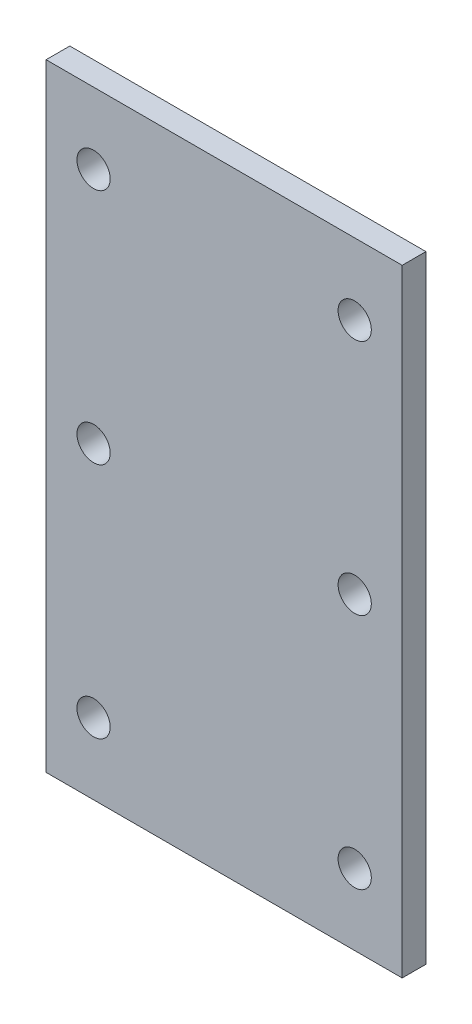
SolidWorks part; units mm, degrees
material "Q235B"
ref_plane "Front Plane" through (0, 0, 0) normal (0, 0, 1) x (1, 0, 0)
ref_plane "Top Plane" through (0, 0, 0) normal (0, 1, 0) x (1, 0, 0)
ref_plane "Right Plane" through (0, 0, 0) normal (1, 0, 0) x (0, 0, -1)
sketch "Sketch1" plane through (0, 0, 0) normal (0, 0, 1) x (1, 0, 0)
  line L1 (75, -130) -> (-75, -130)
  line L2 (75, -130) -> (75, 130)
  line L3 (75, 130) -> (-75, 130)
  line L4 (-75, -130) -> (-75, 130)
  line L5 (75, -130) -> (-75, 130) construction
  line L6 (75, 130) -> (-75, -130) construction
  point P0 (0, 0)
  dimension "D1" = 260
  dimension "D2" = 150
extrude "Boss-Extrude1" add sketch "Sketch1" along normal blind 10
hole_wizard "Ø14.0 (14) Diameter Hole1" positions "Sketch2" profile "Sketch3" hole size "Ø14.0" standard "GB" end condition up to next
sketch "Sketch2" plane through (0, 0, 10) normal (0, 0, 1) x (1, 0, 0)
  line L0 (0, 60.7971) -> (0, 0) construction
  line L1 (0, 0) -> (-55, 0) construction
  line L3 (75, 130) -> (-75, 130) construction
  point P0 (-55, 100)
  point P2 (-55, 0)
  point P15 (-55, -100)
  point P16 (55, -100)
  point P17 (55, 0)
  point P18 (55, 100)
  dimension "D1" = 110
  dimension "D2" = 30
sketch "Sketch3" plane through (-55, 100, 10) normal (1, 0, 0) x (0, -1, 0)
  line L0 (0, 0) -> (0, 10)
  line L1 (0, 10) -> (7, 10)
  line L2 (7, 10) -> (7, 0)
  line L5 (7, 0) -> (0, 0)
  line L11 (0, -6.35) -> (0, 107.95) construction
  dimension "通孔孔直径" = 14
  dimension "通孔孔深度" = 10
